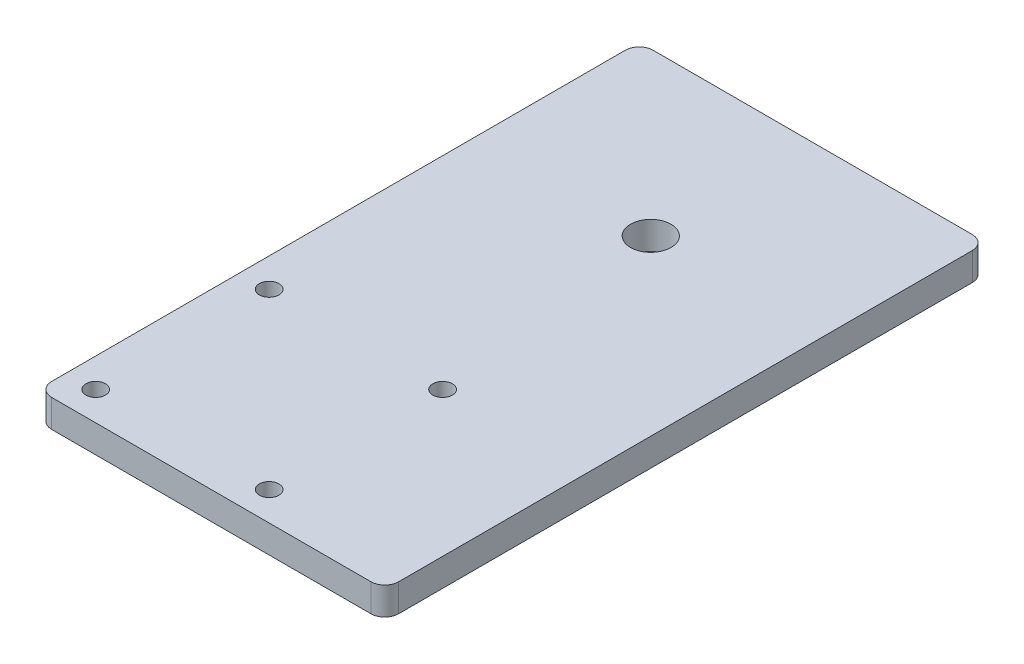
from build123d import *

# Parameters (mm, degrees)
SKETCH_1_W              = 150
SKETCH_1_H              = 260
EXTRUDE_1_DEPTH         = 12
FILLET_1_R              = 6
HOLE_WIZARD_M20_1_D     = 17.5
HOLE_WIZARD_M20_1_DEPTH = 47.5
HOLE_WIZARD_M20_1_TIP   = 5.257530416
HOLE_WIZARD_M10_1_D     = 8.5
HOLE_WIZARD_M10_1_DEPTH = 24.5
HOLE_WIZARD_M10_1_TIP   = 2.553657631


with BuildPart() as part:
    # 草图1 → 凸台-拉伸1 (new body)
    with BuildSketch(Plane(origin=(0, 0, 0), x_dir=(1, 0, 0), z_dir=(0, 1, 0))):
        Rectangle(SKETCH_1_W, SKETCH_1_H)
    extrude(amount=EXTRUDE_1_DEPTH)

    # 圆角1
    fillet_1_edges = [part.edges().sort_by_distance(p)[0] for p in [
        (75, 6, 130),
        (-75, 6, 130),
        (-75, 6, -130),
        (75, 6, -130),
    ]]
    fillet(fillet_1_edges, radius=FILLET_1_R)

    # M20 螺纹孔1
    with Locations(Plane(origin=(0, 0, 0), x_dir=(-1, 0, 0), z_dir=(0, -1, 0))):
        with Locations((0, 60)):
            Hole(HOLE_WIZARD_M20_1_D / 2, depth=HOLE_WIZARD_M20_1_DEPTH)
            with Locations((0, 0, -(HOLE_WIZARD_M20_1_DEPTH + HOLE_WIZARD_M20_1_TIP / 2))):  # 118° drill point
                Cone(0, HOLE_WIZARD_M20_1_D / 2, HOLE_WIZARD_M20_1_TIP, mode=Mode.SUBTRACT)

    # M10 螺纹孔1
    with Locations(Plane(origin=(0, 0, 0), x_dir=(-1, 0, 0), z_dir=(0, -1, 0))):
        with Locations((62.5, -117.5), (62.5, -42.5), (-12.5, -42.5), (-12.5, -117.5)):
            Hole(HOLE_WIZARD_M10_1_D / 2, depth=HOLE_WIZARD_M10_1_DEPTH)
            with Locations((0, 0, -(HOLE_WIZARD_M10_1_DEPTH + HOLE_WIZARD_M10_1_TIP / 2))):  # 118° drill point
                Cone(0, HOLE_WIZARD_M10_1_D / 2, HOLE_WIZARD_M10_1_TIP, mode=Mode.SUBTRACT)


solid = part.part
